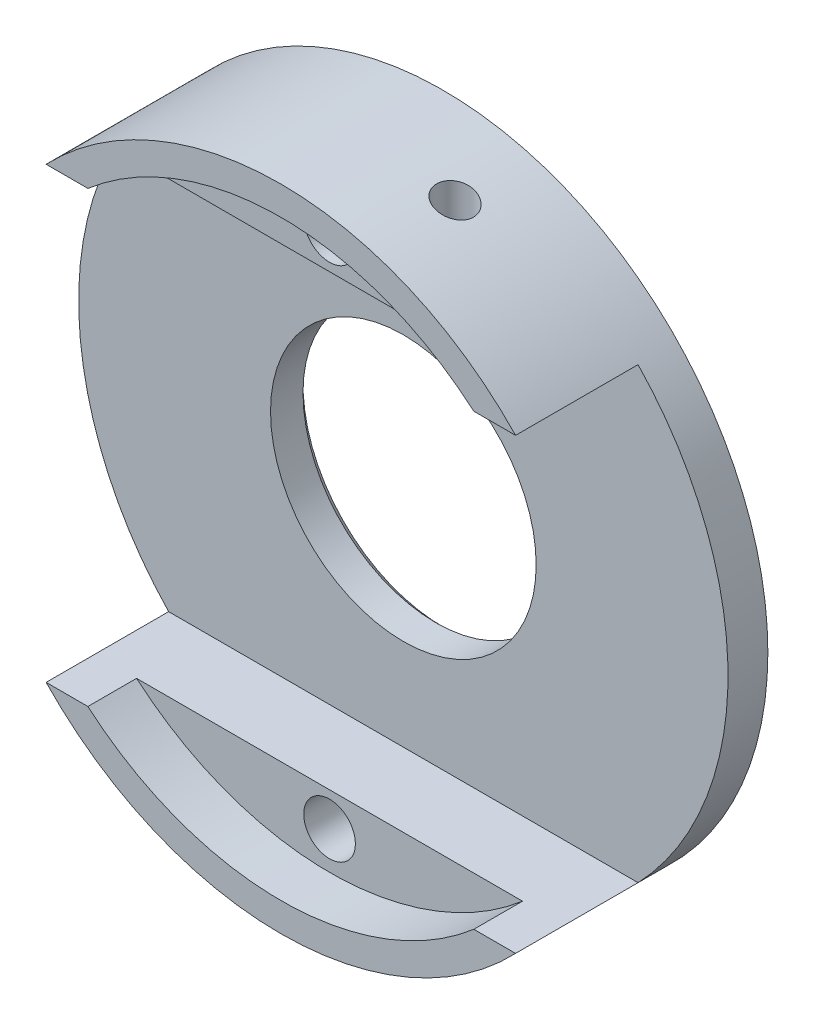
SolidWorks part; units mm, degrees
ref_plane "Front Plane" through (0, 0, 0) normal (0, 0, 1) x (1, 0, 0)
ref_plane "Top Plane" through (0, 0, 0) normal (0, 1, 0) x (1, 0, 0)
ref_plane "Right Plane" through (0, 0, 0) normal (1, 0, 0) x (0, 0, -1)
sketch "Sketch1" plane through (0, 0, 0) normal (0, 0, 1) x (1, 0, 0)
  circle A0 centre (0, 0) radius 22
  dimension "D1" = 44
extrude "Boss-Extrude1" add sketch "Sketch1" along normal blind 11
sketch "Sketch2" plane through (0, 0, 11) normal (0, 0, 1) x (1, 0, 0)
  circle A0 centre (0, 0) radius 20.05
  dimension "D1" = 40.1
extrude "Cut-Extrude1" cut sketch "Sketch2" against normal blind 8.3
sketch "Sketch3" plane through (0, 0, 2.7) normal (0, 0, 1) x (1, 0, 0)
  line L1 (-33.8414, 15.2) -> (33.8414, 15.2)
  line L2 (-33.8414, 15.2) -> (-33.8414, -15.2)
  line L3 (-33.8414, -15.2) -> (33.8414, -15.2)
  line L4 (33.8414, 15.2) -> (33.8414, -15.2)
  line L5 (-33.8414, 15.2) -> (33.8414, -15.2) construction
  line L6 (-33.8414, -15.2) -> (33.8414, 15.2) construction
  point P0 (0, 0)
  dimension "D1" = 30.4
extrude "Cut-Extrude2" cut sketch "Sketch3" along normal up to surface (8.3 mm away) up to face at (20.05, 0, 11)
sketch "Sketch4" plane through (0, 0, 0) normal (0, 0, -1) x (-1, 0, 0)
  circle A0 centre (0, 0) radius 17.5 construction
  circle A1 centre (0, 17.5) radius 1.75
  dimension "D1" = 35
  dimension "D2" = 3.5
extrude "Cut-Extrude3" cut sketch "Sketch4" against normal blind 5
pattern_circular "CirPattern1" count 2 over 360 about axis through (0, 0, 0) along (0, 0, 1) of "Cut-Extrude3"
sketch "Sketch5" plane through (0, 0, 0) normal (0, 0, -1) x (-1, 0, 0)
  circle A0 centre (0, 0) radius 9
  dimension "D1" = 18
extrude "Cut-Extrude4" cut sketch "Sketch5" against normal up to next
chamfer "Chamfer1" distance 1.5 angle 45 2 edges at (1.75, -17.5, 0) (-1.75, 17.5, 0)
chamfer "Chamfer2" distance 0.5 angle 45 1 edges at (-9, 0, 0)
sketch "Sketch6" plane through (0, 0, 11) normal (0, 0, 1) x (1, 0, 0)
  line L1 (-45.4761, 23.5) -> (45.4761, 23.5)
  line L2 (-45.4761, 23.5) -> (-45.4761, -23.5)
  line L3 (-45.4761, -23.5) -> (45.4761, -23.5)
  line L4 (45.4761, 23.5) -> (45.4761, -23.5)
  line L5 (-45.4761, 23.5) -> (45.4761, -23.5) construction
  line L6 (-45.4761, -23.5) -> (45.4761, 23.5) construction
  point P0 (0, 0)
  dimension "D1" = 47
extrude "Cut-Extrude5" cut sketch "Sketch6" against normal up to next (8.3 mm away) flip side to cut
sketch "Sketch7" plane through (0, 0, 2.7) normal (0, 0, 1) x (1, 0, 0)
  line L0 (-13.0753, 15.2) -> (13.0753, 15.2)
  line L1 (-13.0753, -15.2) -> (13.0753, -15.2)
  circle A0 centre (0, -17.5) radius 1.75 construction
  circle A1 centre (0, 17.5) radius 1.75 construction
  arc A2 (-13.0753, -15.2) -> (13.0753, -15.2) centre (0, 0) ccw construction
  arc A3 (13.0753, 15.2) -> (-13.0753, 15.2) centre (0, 0) ccw construction
  circle A4 centre (0, -17.5) radius 1.75
  circle A5 centre (0, 17.5) radius 1.75
  arc A6 (-13.0753, -15.2) -> (13.0753, -15.2) centre (0, 0) ccw
  arc A7 (13.0753, 15.2) -> (-13.0753, 15.2) centre (0, 0) ccw
extrude "Boss-Extrude2" add sketch "Sketch7" along normal blind 5
sketch "Sketch8" plane through (0, 15.2, 0) normal (0, -1, 0) x (1, 0, 0)
  line L0 (0, 7.7) -> (0, 2.7) construction
  line L1 (13.0753, 7.7) -> (-13.0753, 7.7) construction
  line L2 (-15.9047, 2.7) -> (15.9047, 2.7) construction
  line L3 (0, 5.2) -> (6, 5.2) construction
  circle A0 centre (6, 5.2) radius 1.25
  dimension "D2" = 2.5
  dimension "D1" = 6
extrude "Cut-Extrude6" cut sketch "Sketch8" against normal blind 11
cosmetic thread "Cosmetic Thread1" parameters "D2"=3
